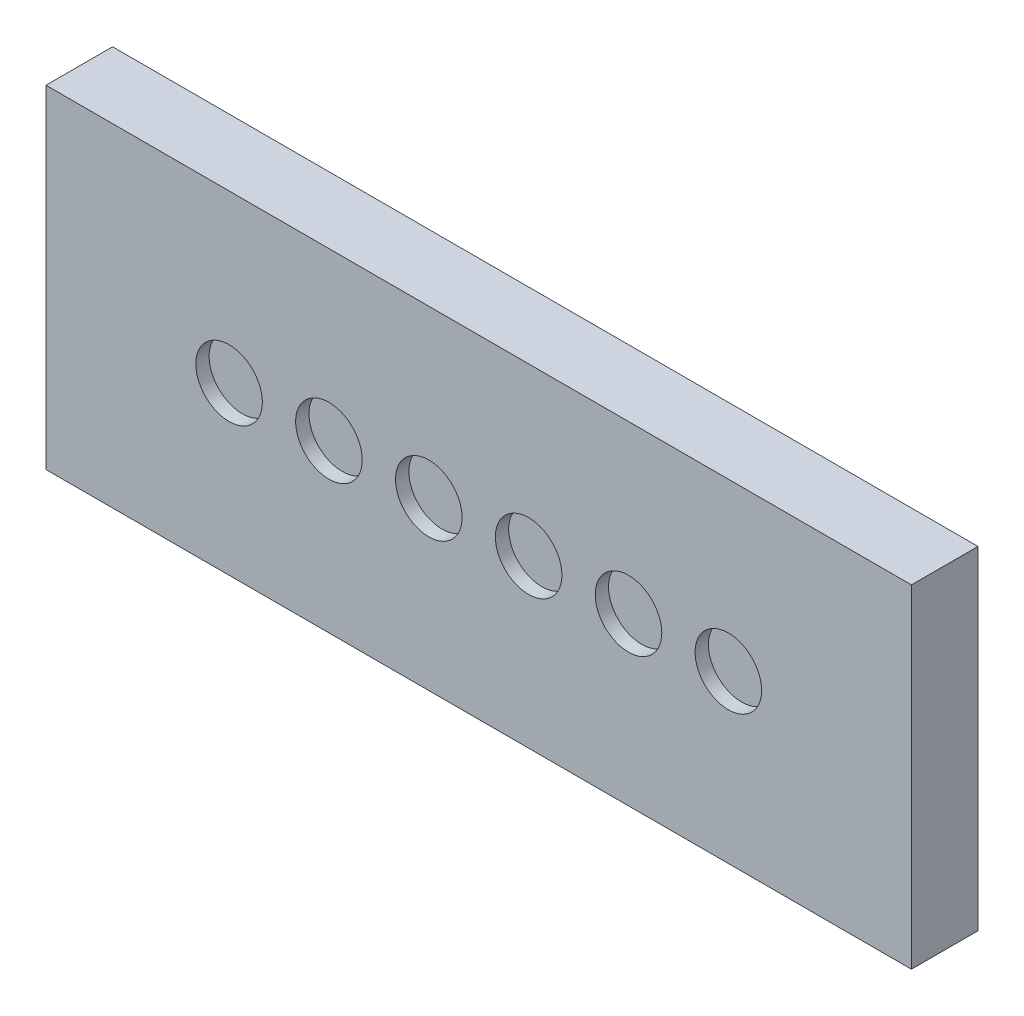
SolidWorks part; units mm, degrees
ref_plane "Front Plane" through (0, 0, 0) normal (0, 0, 1) x (1, 0, 0)
ref_plane "Top Plane" through (0, 0, 0) normal (0, 1, 0) x (1, 0, 0)
ref_plane "Right Plane" through (0, 0, 0) normal (1, 0, 0) x (0, 0, -1)
other "Configuration Table"
sketch "Sketch1" plane through (0, 0, 0) normal (0, 0, 1) x (1, 0, 0)
  line L1 (65, -25) -> (-65, -25)
  line L2 (65, -25) -> (65, 25)
  line L3 (65, 25) -> (-65, 25)
  line L4 (-65, -25) -> (-65, 25)
  line L5 (65, -25) -> (-65, 25) construction
  line L6 (65, 25) -> (-65, -25) construction
  point P0 (0, 0)
  dimension "D1" = 130
  dimension "D2" = 50
extrude "Boss-Extrude1" add sketch "Sketch1" along normal blind 10
sketch "Sketch2" plane through (0, 0, 10) normal (0, 0, 1) x (1, 0, 0)
  line L0 (-65, 0) -> (65, 0) construction
  line L1 (-65, 25) -> (-65, -25) construction
  line L2 (65, -25) -> (65, 25) construction
  circle A0 centre (-37.5, 0) radius 5
  circle A1 centre (-22.5, 0) radius 5
  circle A2 centre (-7.5, 0) radius 5
  circle A3 centre (7.5, 0) radius 5
  circle A4 centre (22.5, 0) radius 5
  circle A5 centre (37.5, 0) radius 5
  dimension "D1" = 10
  dimension "D2" = 27.5
  dimension "D3" = 6
extrude "Cut-Extrude1" cut sketch "Sketch2" against normal blind 2
